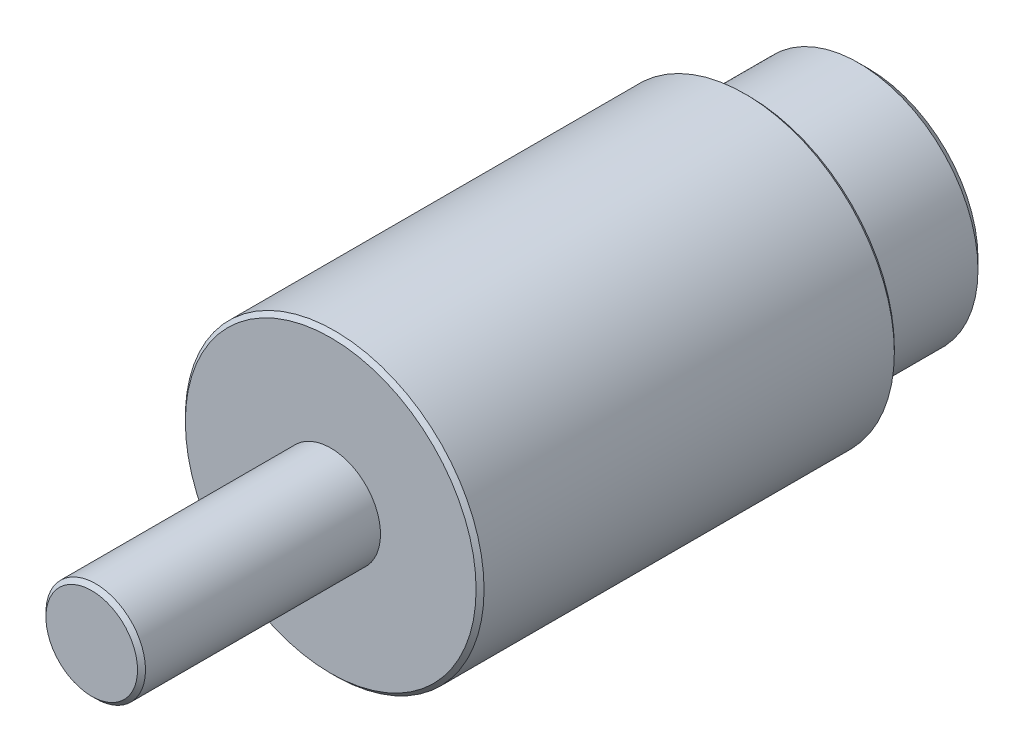
SolidWorks part; units mm, degrees
ref_plane "主视基准图" through (0, 0, 0) normal (0, 0, 1) x (1, 0, 0)
ref_plane "上视基准图" through (0, 0, 0) normal (0, 1, 0) x (1, 0, 0)
ref_plane "右视基准图" through (0, 0, 0) normal (1, 0, 0) x (0, 0, -1)
sketch "草图1" plane through (0, 0, 0) normal (0, 0, 1) x (1, 0, 0)
  circle A0 centre (0, 0) radius 6
  dimension "D1" = 12
extrude "凸台-拉伸1" add sketch "草图1" along normal mid plane 27
chamfer "倒角1" distance 0.5 angle 45 2 edges at (6, 0, -13.5) (6, 0, 13.5)
sketch "草图2" plane through (0, 0, 13.5) normal (0, 0, 1) x (1, 0, 0)
  circle A0 centre (0, 0) radius 2.5
  dimension "D1" = 5
extrude "凸台-拉伸2" add sketch "草图2" along normal blind 12
chamfer "倒角2" distance 0.2 angle 45 1 edges at (2.5, 0, 25.5)
sketch "草图3" plane through (0, 0, 13.5) normal (0, 0, 1) x (1, 0, 0)
  circle A0 centre (0, 0) radius 7.5
  dimension "D1" = 15
extrude "凸台-拉伸3" add sketch "草图3" against normal blind 21
cosmetic thread "装饰螺纹线2" parameters "D2"=14
chamfer "倒角3" distance 0.2 angle 45 2 edges at (7.5, 0, -7.5) (7.5, 0, 13.5)
